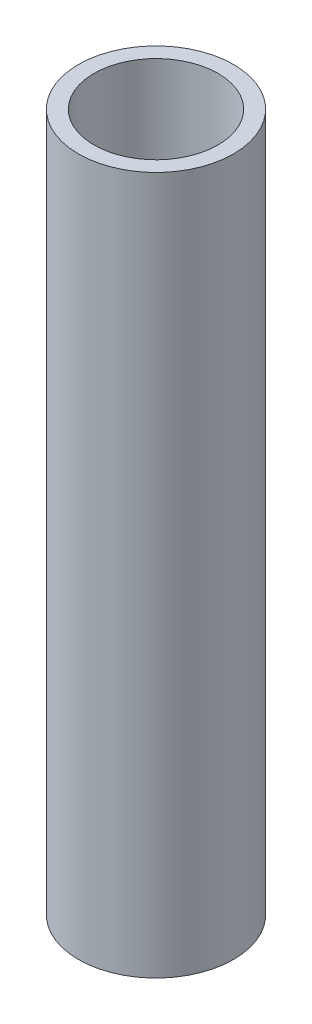
from build123d import *

# Parameters (mm, degrees)
SKETCH11_R                             = 10
SKETCH11_R_2                           = 8
GB_T_6728_2002_ROUND_TUBE_20_2_1_DEPTH = 90


with BuildPart() as part:
    # Sketch11 → GB/T 6728-2002 round tube 20 × 2(1) (new body)
    with BuildSketch(Plane(origin=(0, 0, 0), x_dir=(-1, 0, 0), z_dir=(0, 1, 0))):
        Circle(SKETCH11_R)
        Circle(SKETCH11_R_2, mode=Mode.SUBTRACT)
    extrude(amount=GB_T_6728_2002_ROUND_TUBE_20_2_1_DEPTH)


solid = part.part
